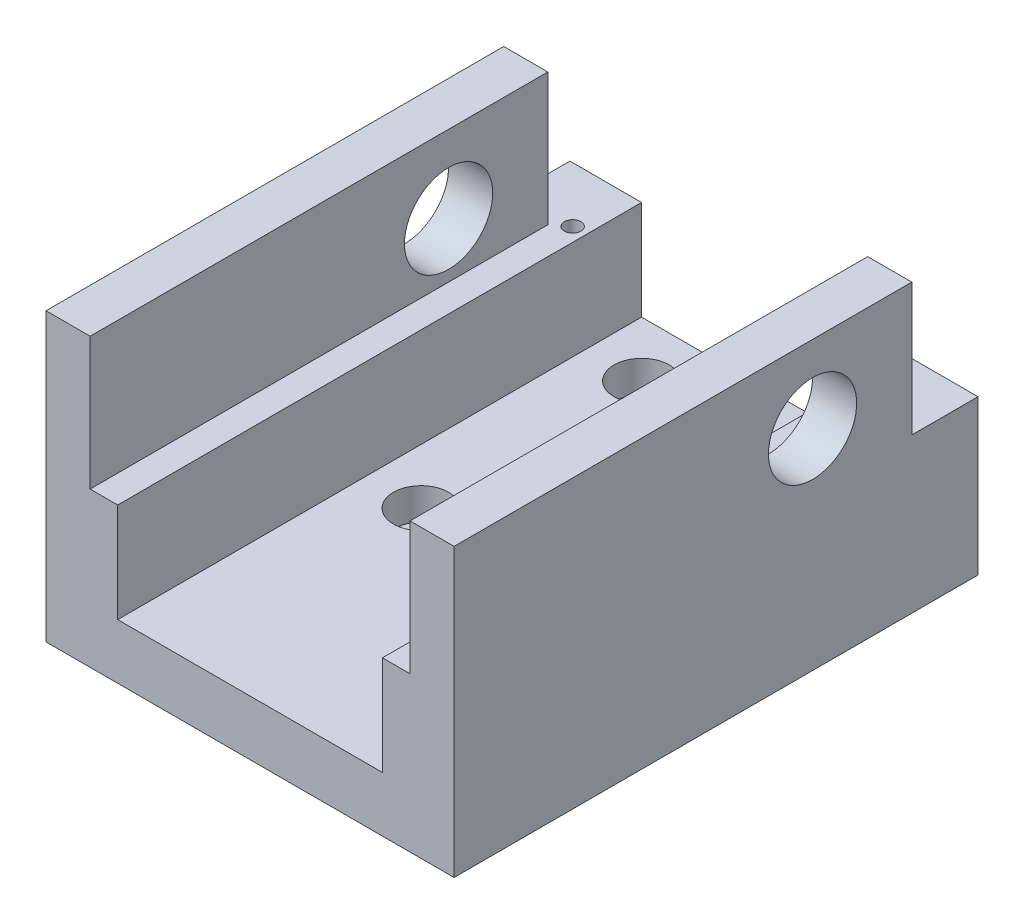
SolidWorks part; units mm, degrees
ref_plane "前视基准面" through (0, 0, 0) normal (0, 0, 1) x (1, 0, 0)
ref_plane "上视基准面" through (0, 0, 0) normal (0, 1, 0) x (1, 0, 0)
ref_plane "右视基准面" through (0, 0, 0) normal (1, 0, 0) x (0, 0, -1)
sketch "草图1" plane through (0, 0, 0) normal (0, 0, 1) x (1, 0, 0)
  line L0 (-42.9661, 24) -> (-42.9661, -28)
  line L1 (-42.9661, -28) -> (31.0339, -28)
  line L2 (31.0339, -28) -> (31.0339, 24)
  line L3 (-42.9661, 24) -> (-34.9661, 24)
  line L4 (-34.9661, 24) -> (-34.9661, 0)
  line L5 (-34.9661, 0) -> (-29.9661, 0)
  line L6 (-29.9661, 0) -> (-29.9661, -18)
  line L7 (-29.9661, -18) -> (18.0339, -18)
  line L8 (18.0339, -18) -> (18.0339, 0)
  line L9 (18.0339, 0) -> (23.0339, 0)
  line L10 (23.0339, 0) -> (23.0339, 24)
  line L11 (23.0339, 24) -> (31.0339, 24)
  dimension "D1" = 52
  dimension "D2" = 74
  dimension "D3" = 8
  dimension "D4" = 24
  dimension "D5" = 5
  dimension "D6" = 8
  dimension "D7" = 24
  dimension "D8" = 5
  dimension "D9" = 18
extrude "凸台-拉伸1" add sketch "草图1" along normal blind 95
sketch "草图2" plane through (0, -18, 0) normal (0, 1, 0) x (1, 0, 0)
  line L0 (18.0339, 0) -> (-29.9661, 0) construction
  line L1 (-29.9661, -95) -> (-29.9661, 0) construction
  line L2 (-29.9661, -95) -> (-29.9661, 0) construction
  line L3 (18.0339, -95) -> (18.0339, 0) construction
  line L4 (18.0339, -95) -> (18.0339, 0) construction
  circle A0 centre (-19.9661, -10) radius 2.75
  circle A1 centre (-19.9661, -50) radius 2.75
  circle A2 centre (8.0339, -10) radius 2.75
  circle A3 centre (8.0339, -50) radius 2.75
  dimension "D9" = 5.5
  dimension "D10" = 5.5
  dimension "D11" = 5.5
  dimension "D12" = 5.5
  dimension "D1" = 10
  dimension "D2" = 10
  dimension "D3" = 10
  dimension "D4" = 50
  dimension "D5" = 10
  dimension "D6" = 10
  dimension "D7" = 50
  dimension "D8" = 10
extrude "切除-拉伸1" cut sketch "草图2" against normal through all
sketch "草图3" plane through (0, -18, 0) normal (0, 1, 0) x (1, 0, 0)
  circle A0 centre (-19.9661, -10) radius 5
  circle A1 centre (-19.9661, -50) radius 5
  circle A2 centre (8.0339, -10) radius 5
  circle A3 centre (8.0339, -50) radius 5
  dimension "D1" = 10
  dimension "D2" = 10
  dimension "D3" = 10
  dimension "D4" = 10
extrude "切除-拉伸2" cut sketch "草图3" against normal blind 5.75
sketch "草图4" plane through (-42.9661, 0, 0) normal (-1, 0, 0) x (0, 0, 1)
  line L0 (0, 0) -> (12, 0)
  line L1 (0, 24) -> (0, -28) construction
  line L2 (12, 0) -> (12, 24)
  line L3 (95, 24) -> (0, 24) construction
  line L4 (12, 24) -> (0, 24)
  line L5 (0, 24) -> (0, 0)
  dimension "D1" = 12
  dimension "D2" = 24
extrude "切除-拉伸3" cut sketch "草图4" against normal through all
sketch "草图5" plane through (0, 0, 0) normal (0, 1, 0) x (1, 0, 0)
  line L0 (-29.9661, 0) -> (-42.9661, 0) construction
  line L1 (-42.9661, 0) -> (-42.9661, -12) construction
  line L2 (31.0339, 0) -> (18.0339, 0) construction
  line L3 (31.0339, 0) -> (31.0339, -12) construction
  circle A0 centre (-32.4661, -10) radius 1.25
  circle A1 centre (20.5339, -10) radius 1.25
  dimension "D5" = 2.5
  dimension "D6" = 2.5
  dimension "D1" = 10
  dimension "D2" = 10.5
  dimension "D3" = 10
  dimension "D4" = 10.5
extrude "切除-拉伸4" cut sketch "草图5" against normal blind 7.5
sketch "草图6" plane through (0, 0, 0) normal (0, 1, 0) x (1, 0, 0)
  circle A0 centre (-32.4661, -10) radius 1.5
  circle A1 centre (20.5339, -10) radius 1.5
  dimension "D1" = 3
  dimension "D2" = 3
extrude "切除-拉伸5" cut sketch "草图6" against normal blind 6
sketch "草图7" plane through (-42.9661, 0, 0) normal (-1, 0, 0) x (0, 0, 1)
  line L0 (95, 24) -> (12, 24) construction
  line L1 (12, 0) -> (12, 24) construction
  circle A0 centre (30, 10) radius 8
  dimension "D1" = 16
  dimension "D2" = 14
  dimension "D3" = 18
extrude "切除-拉伸6" cut sketch "草图7" against normal through all
